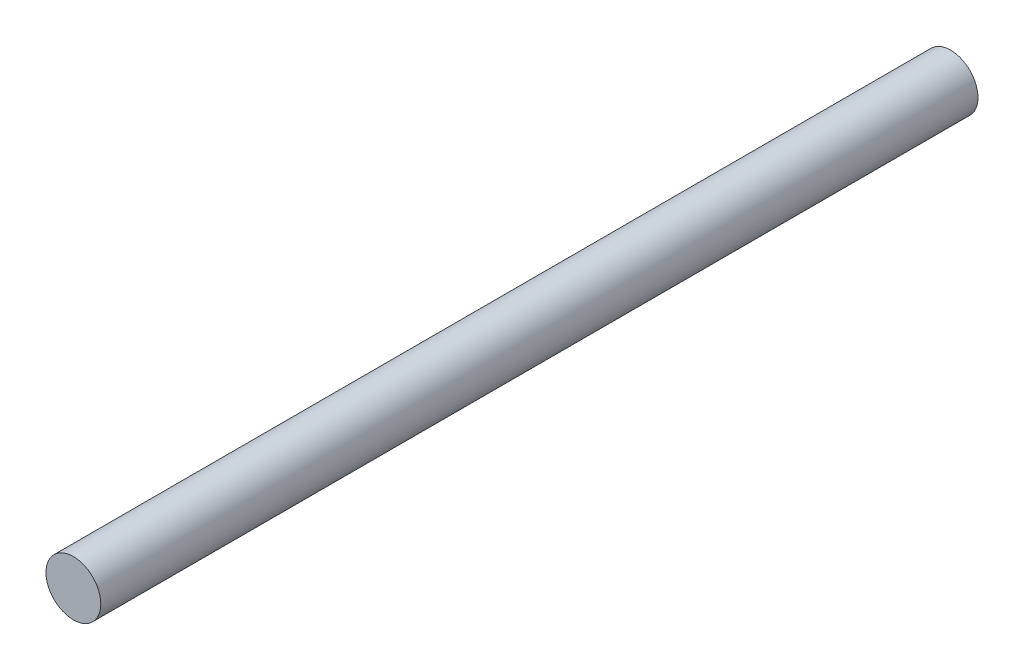
SolidWorks part; units mm, degrees
ref_plane "前视基准面" through (0, 0, 0) normal (0, 0, 1) x (1, 0, 0)
ref_plane "上视基准面" through (0, 0, 0) normal (0, 1, 0) x (1, 0, 0)
ref_plane "右视基准面" through (0, 0, 0) normal (1, 0, 0) x (0, 0, -1)
sketch "草图1" plane through (0, 0, 0) normal (0, 0, 1) x (1, 0, 0)
  circle A0 centre (0, 0) radius 7.5
  dimension "D1" = 15
extrude "凸台-拉伸1" add sketch "草图1" along normal blind 240
